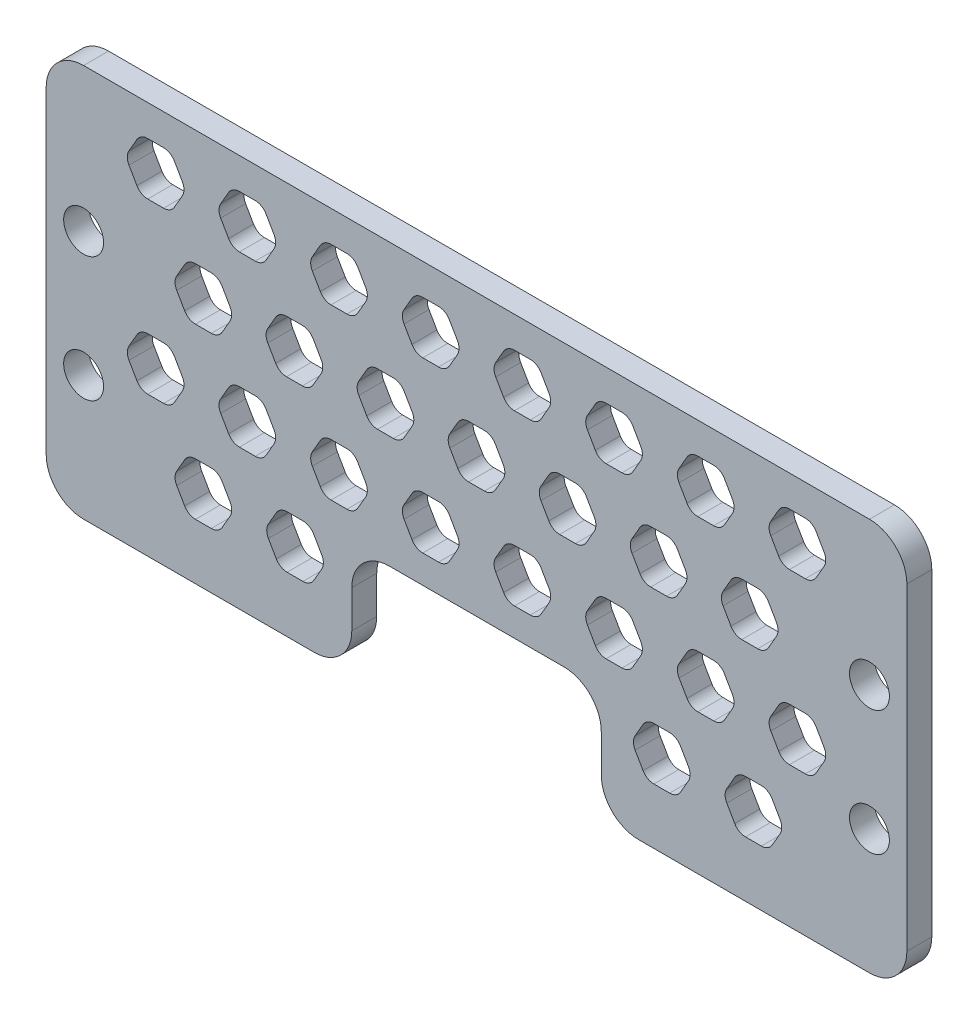
from build123d import *

# Parameters (mm, degrees)
SKETCH1_R              = 1.6
BOSS_EXTRUDE1_DEPTH    = 2
CUT_EXTRUDE1_DEPTH     = 38.977789562
R1_CUTOUT_FILLET_R     = 1
R3_OUTER_EDGE_FILLET_R = 3


with BuildPart() as part:
    # Sketch1 → Boss-Extrude1 (new body)
    with BuildSketch(Plane.XY):
        Polygon((-34.5, 15.75), (34.5, 15.75), (34.5, -15.75), (10, -15.75), (10, -6.75), (-10, -6.75), (-10, -15.75), (-34.5, -15.75), align=None)
        with Locations((-31.5, 4.25)):
            Circle(SKETCH1_R, mode=Mode.SUBTRACT)
        with Locations((-31.5, -5.75)):
            Circle(SKETCH1_R, mode=Mode.SUBTRACT)
        with Locations(Location((31.5, -5.75, 0), (0, 0, 180))):
            Circle(SKETCH1_R, mode=Mode.SUBTRACT)
        with Locations(Location((31.5, 4.25, 0), (0, 0, 180))):
            Circle(SKETCH1_R, mode=Mode.SUBTRACT)
    extrude(amount=BOSS_EXTRUDE1_DEPTH)

    # Sketch2 → Cut-Extrude1 (cut, through all)
    with BuildSketch(Plane.XY.offset(2)):
        Polygon((-28.148969045, 11.15), (-26.936533479, 13.25), (-24.511662349, 13.25), (-23.299226784, 11.15), (-24.511662349, 9.05), (-26.936533479, 9.05), align=None)
        Polygon((-19.586791218, 9.05), (-20.799226784, 11.15), (-19.586791218, 13.25), (-17.161920088, 13.25), (-15.949484522, 11.15), (-17.161920088, 9.05), align=None)
        Polygon((-12.237048957, 9.05), (-13.449484522, 11.15), (-12.237048957, 13.25), (-9.812177826, 13.25), (-8.599742261, 11.15), (-9.812177826, 9.05), align=None)
        Polygon((-4.887306696, 9.05), (-6.099742261, 11.15), (-4.887306696, 13.25), (-2.462435565, 13.25), (-1.25, 11.15), (-2.462435565, 9.05), align=None)
        Polygon((2.462435565, 9.05), (1.25, 11.15), (2.462435565, 13.25), (4.887306696, 13.25), (6.099742261, 11.15), (4.887306696, 9.05), align=None)
        Polygon((9.812177826, 9.05), (8.599742261, 11.15), (9.812177826, 13.25), (12.237048957, 13.25), (13.449484522, 11.15), (12.237048957, 9.05), align=None)
        Polygon((17.161920088, 9.05), (15.949484522, 11.15), (17.161920088, 13.25), (19.586791218, 13.25), (20.799226784, 11.15), (19.586791218, 9.05), align=None)
        Polygon((24.511662349, 9.05), (23.299226784, 11.15), (24.511662349, 13.25), (26.936533479, 13.25), (28.148969045, 11.15), (26.936533479, 9.05), align=None)
        Polygon((-24.324097914, 4.374871131), (-23.111662349, 6.474871131), (-20.686791218, 6.474871131), (-19.474355653, 4.374871131), (-20.686791218, 2.274871131), (-23.111662349, 2.274871131), align=None)
        Polygon((-15.811920088, 2.274871131), (-17.024355653, 4.374871131), (-15.811920088, 6.474871131), (-13.387048957, 6.474871131), (-12.174613392, 4.374871131), (-13.387048957, 2.274871131), align=None)
        Polygon((-8.512177826, 2.274871131), (-9.724613392, 4.374871131), (-8.512177826, 6.474871131), (-6.087306696, 6.474871131), (-4.874871131, 4.374871131), (-6.087306696, 2.274871131), align=None)
        Polygon((-1.212435565, 2.274871131), (-2.424871131, 4.374871131), (-1.212435565, 6.474871131), (1.212435565, 6.474871131), (2.424871131, 4.374871131), (1.212435565, 2.274871131), align=None)
        Polygon((6.087306696, 2.274871131), (4.874871131, 4.374871131), (6.087306696, 6.474871131), (8.512177826, 6.474871131), (9.724613392, 4.374871131), (8.512177826, 2.274871131), align=None)
        Polygon((13.387048957, 2.274871131), (12.174613392, 4.374871131), (13.387048957, 6.474871131), (15.811920088, 6.474871131), (17.024355653, 4.374871131), (15.811920088, 2.274871131), align=None)
        Polygon((20.686791218, 2.274871131), (19.474355653, 4.374871131), (20.686791218, 6.474871131), (23.111662349, 6.474871131), (24.324097914, 4.374871131), (23.111662349, 2.274871131), align=None)
        Polygon((-26.936533479, -4.500257739), (-28.148969045, -2.400257739), (-26.936533479, -0.300257739), (-24.511662349, -0.300257739), (-23.299226784, -2.400257739), (-24.511662349, -4.500257739), align=None)
        Polygon((-19.586791218, -4.500257739), (-20.799226784, -2.400257739), (-19.586791218, -0.300257739), (-17.161920088, -0.300257739), (-15.949484522, -2.400257739), (-17.161920088, -4.500257739), align=None)
        Polygon((-12.237048957, -4.500257739), (-13.449484522, -2.400257739), (-12.237048957, -0.300257739), (-9.812177826, -0.300257739), (-8.599742261, -2.400257739), (-9.812177826, -4.500257739), align=None)
        Polygon((-4.887306696, -4.500257739), (-6.099742261, -2.400257739), (-4.887306696, -0.300257739), (-2.462435565, -0.300257739), (-1.25, -2.400257739), (-2.462435565, -4.500257739), align=None)
        Polygon((2.462435565, -4.500257739), (1.25, -2.400257739), (2.462435565, -0.300257739), (4.887306696, -0.300257739), (6.099742261, -2.400257739), (4.887306696, -4.500257739), align=None)
        Polygon((9.812177826, -4.500257739), (8.599742261, -2.400257739), (9.812177826, -0.300257739), (12.237048957, -0.300257739), (13.449484522, -2.400257739), (12.237048957, -4.500257739), align=None)
        Polygon((17.161920088, -4.500257739), (15.949484522, -2.400257739), (17.161920088, -0.300257739), (19.586791218, -0.300257739), (20.799226784, -2.400257739), (19.586791218, -4.500257739), align=None)
        Polygon((24.511662349, -4.500257739), (23.299226784, -2.400257739), (24.511662349, -0.300257739), (26.936533479, -0.300257739), (28.148969045, -2.400257739), (26.936533479, -4.500257739), align=None)
        Polygon((-24.324097914, -9.175386608), (-23.111662349, -7.075386608), (-20.686791218, -7.075386608), (-19.474355653, -9.175386608), (-20.686791218, -11.275386608), (-23.111662349, -11.275386608), align=None)
        Polygon((-15.761920088, -11.275386608), (-16.974355653, -9.175386608), (-15.761920088, -7.075386608), (-13.337048957, -7.075386608), (-12.124613392, -9.175386608), (-13.337048957, -11.275386608), align=None)
        Polygon((13.637048957, -11.275386608), (12.424613392, -9.175386608), (13.637048957, -7.075386608), (16.061920088, -7.075386608), (17.274355653, -9.175386608), (16.061920088, -11.275386608), align=None)
        Polygon((20.986791218, -11.275386608), (19.774355653, -9.175386608), (20.986791218, -7.075386608), (23.411662349, -7.075386608), (24.624097914, -9.175386608), (23.411662349, -11.275386608), align=None)
    extrude(amount=-CUT_EXTRUDE1_DEPTH, mode=Mode.SUBTRACT)

    # R1 cutout fillet
    r1_cutout_fillet_edges = [part.edges().sort_by_distance(p)[0] for p in [
        (-28.148969045, -2.400257739, 1),
        (-26.936533479, -0.300257739, 1),
        (-24.511662349, -0.300257739, 1),
        (-23.299226784, -2.400257739, 1),
        (-24.511662349, -4.500257739, 1),
        (-26.936533479, -4.500257739, 1),
        (-17.024355653, 4.374871131, 1),
        (-15.811920088, 6.474871131, 1),
        (-13.387048957, 6.474871131, 1),
        (-12.174613392, 4.374871131, 1),
        (-13.387048957, 2.274871131, 1),
        (-15.811920088, 2.274871131, 1),
        (-9.724613392, 4.374871131, 1),
        (-8.512177826, 6.474871131, 1),
        (-6.087306696, 6.474871131, 1),
        (-4.874871131, 4.374871131, 1),
        (-6.087306696, 2.274871131, 1),
        (-8.512177826, 2.274871131, 1),
        (-2.424871131, 4.374871131, 1),
        (-1.212435565, 6.474871131, 1),
        (1.212435565, 6.474871131, 1),
        (2.424871131, 4.374871131, 1),
        (1.212435565, 2.274871131, 1),
        (-1.212435565, 2.274871131, 1),
        (-20.799226784, -2.400257739, 1),
        (-19.586791218, -0.300257739, 1),
        (-17.161920088, -0.300257739, 1),
        (-15.949484522, -2.400257739, 1),
        (-17.161920088, -4.500257739, 1),
        (-19.586791218, -4.500257739, 1),
        (19.474355653, 4.374871131, 1),
        (20.686791218, 6.474871131, 1),
        (23.111662349, 6.474871131, 1),
        (24.324097914, 4.374871131, 1),
        (23.111662349, 2.274871131, 1),
        (20.686791218, 2.274871131, 1),
        (12.174613392, 4.374871131, 1),
        (13.387048957, 6.474871131, 1),
        (15.811920088, 6.474871131, 1),
        (17.024355653, 4.374871131, 1),
        (15.811920088, 2.274871131, 1),
        (13.387048957, 2.274871131, 1),
        (4.874871131, 4.374871131, 1),
        (6.087306696, 6.474871131, 1),
        (8.512177826, 6.474871131, 1),
        (9.724613392, 4.374871131, 1),
        (8.512177826, 2.274871131, 1),
        (6.087306696, 2.274871131, 1),
        (-20.799226784, 11.15, 1),
        (-19.586791218, 13.25, 1),
        (-17.161920088, 13.25, 1),
        (-15.949484522, 11.15, 1),
        (-17.161920088, 9.05, 1),
        (-19.586791218, 9.05, 1),
        (-13.449484522, 11.15, 1),
        (-12.237048957, 13.25, 1),
        (-9.812177826, 13.25, 1),
        (-8.599742261, 11.15, 1),
        (-9.812177826, 9.05, 1),
        (-12.237048957, 9.05, 1),
        (-6.099742261, 11.15, 1),
        (-4.887306696, 13.25, 1),
        (-2.462435565, 13.25, 1),
        (-1.25, 11.15, 1),
        (-2.462435565, 9.05, 1),
        (-4.887306696, 9.05, 1),
        (1.25, 11.15, 1),
        (2.462435565, 13.25, 1),
        (4.887306696, 13.25, 1),
        (6.099742261, 11.15, 1),
        (4.887306696, 9.05, 1),
        (2.462435565, 9.05, 1),
        (-23.111662349, 2.274871131, 1),
        (-24.324097914, 4.374871131, 1),
        (-23.111662349, 6.474871131, 1),
        (-20.686791218, 6.474871131, 1),
        (-19.474355653, 4.374871131, 1),
        (-20.686791218, 2.274871131, 1),
        (23.299226784, 11.15, 1),
        (24.511662349, 13.25, 1),
        (26.936533479, 13.25, 1),
        (28.148969045, 11.15, 1),
        (26.936533479, 9.05, 1),
        (24.511662349, 9.05, 1),
        (15.949484522, 11.15, 1),
        (17.161920088, 13.25, 1),
        (19.586791218, 13.25, 1),
        (20.799226784, 11.15, 1),
        (19.586791218, 9.05, 1),
        (17.161920088, 9.05, 1),
        (8.599742261, 11.15, 1),
        (9.812177826, 13.25, 1),
        (12.237048957, 13.25, 1),
        (13.449484522, 11.15, 1),
        (12.237048957, 9.05, 1),
        (9.812177826, 9.05, 1),
        (19.774355653, -9.175386608, 1),
        (20.986791218, -7.075386608, 1),
        (23.411662349, -7.075386608, 1),
        (24.624097914, -9.175386608, 1),
        (23.411662349, -11.275386608, 1),
        (20.986791218, -11.275386608, 1),
        (12.424613392, -9.175386608, 1),
        (13.637048957, -7.075386608, 1),
        (16.061920088, -7.075386608, 1),
        (17.274355653, -9.175386608, 1),
        (16.061920088, -11.275386608, 1),
        (13.637048957, -11.275386608, 1),
        (-13.449484522, -2.400257739, 1),
        (-12.237048957, -0.300257739, 1),
        (-9.812177826, -0.300257739, 1),
        (-8.599742261, -2.400257739, 1),
        (-9.812177826, -4.500257739, 1),
        (-12.237048957, -4.500257739, 1),
        (-6.099742261, -2.400257739, 1),
        (-4.887306696, -0.300257739, 1),
        (-2.462435565, -0.300257739, 1),
        (-1.25, -2.400257739, 1),
        (-2.462435565, -4.500257739, 1),
        (-4.887306696, -4.500257739, 1),
        (1.25, -2.400257739, 1),
        (2.462435565, -0.300257739, 1),
        (4.887306696, -0.300257739, 1),
        (6.099742261, -2.400257739, 1),
        (4.887306696, -4.500257739, 1),
        (2.462435565, -4.500257739, 1),
        (8.599742261, -2.400257739, 1),
        (9.812177826, -0.300257739, 1),
        (12.237048957, -0.300257739, 1),
        (13.449484522, -2.400257739, 1),
        (12.237048957, -4.500257739, 1),
        (9.812177826, -4.500257739, 1),
        (15.949484522, -2.400257739, 1),
        (17.161920088, -0.300257739, 1),
        (19.586791218, -0.300257739, 1),
        (20.799226784, -2.400257739, 1),
        (19.586791218, -4.500257739, 1),
        (17.161920088, -4.500257739, 1),
        (23.299226784, -2.400257739, 1),
        (24.511662349, -0.300257739, 1),
        (26.936533479, -0.300257739, 1),
        (28.148969045, -2.400257739, 1),
        (26.936533479, -4.500257739, 1),
        (24.511662349, -4.500257739, 1),
        (-23.111662349, -11.275386608, 1),
        (-24.324097914, -9.175386608, 1),
        (-23.111662349, -7.075386608, 1),
        (-20.686791218, -7.075386608, 1),
        (-19.474355653, -9.175386608, 1),
        (-20.686791218, -11.275386608, 1),
        (-16.974355653, -9.175386608, 1),
        (-15.761920088, -7.075386608, 1),
        (-13.337048957, -7.075386608, 1),
        (-12.124613392, -9.175386608, 1),
        (-13.337048957, -11.275386608, 1),
        (-15.761920088, -11.275386608, 1),
        (-26.936533479, 9.05, 1),
        (-28.148969045, 11.15, 1),
        (-26.936533479, 13.25, 1),
        (-24.511662349, 13.25, 1),
        (-23.299226784, 11.15, 1),
        (-24.511662349, 9.05, 1),
    ]]
    fillet(r1_cutout_fillet_edges, radius=R1_CUTOUT_FILLET_R)

    # R3 outer edge fillet
    r3_outer_edge_fillet_edges = [part.edges().sort_by_distance(p)[0] for p in [
        (10, -15.75, 1),
        (10, -6.75, 1),
        (-10, -6.75, 1),
        (-10, -15.75, 1),
        (-34.5, -15.75, 1),
        (-34.5, 15.75, 1),
        (34.5, 15.75, 1),
        (34.5, -15.75, 1),
    ]]
    fillet(r3_outer_edge_fillet_edges, radius=R3_OUTER_EDGE_FILLET_R)


solid = part.part
